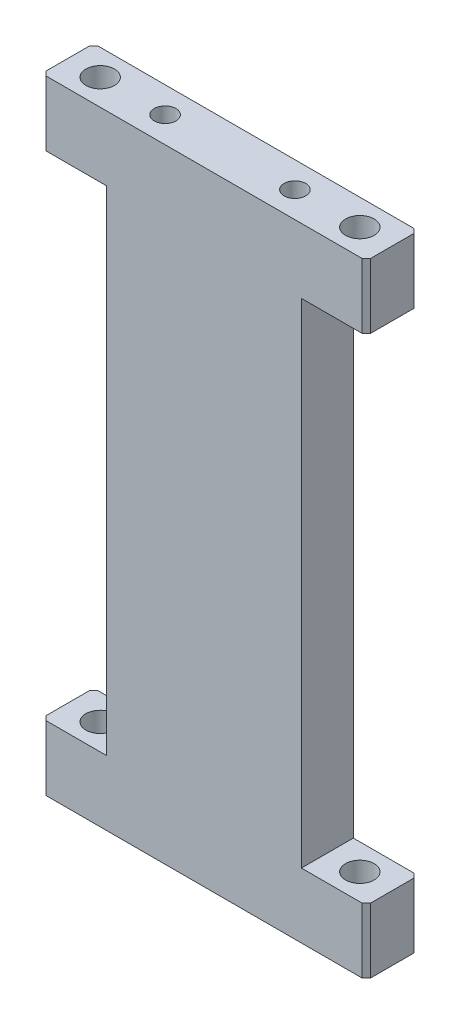
SolidWorks part; units mm, degrees
material "AL6061"
ref_plane "Front Plane" through (0, 0, 0) normal (0, 0, 1) x (1, 0, 0)
ref_plane "Top Plane" through (0, 0, 0) normal (0, 1, 0) x (1, 0, 0)
ref_plane "Right Plane" through (0, 0, 0) normal (1, 0, 0) x (0, 0, -1)
sketch "Sketch1" plane through (0, 0, 0) normal (0, 0, 1) x (1, 0, 0)
  line L1 (-37.5, 72) -> (37.5, 72)
  line L2 (-37.5, 72) -> (-37.5, -72)
  line L3 (-37.5, -72) -> (37.5, -72)
  line L4 (37.5, 72) -> (37.5, -72)
  line L5 (-37.5, 72) -> (37.5, -72) construction
  line L6 (-37.5, -72) -> (37.5, 72) construction
  point P0 (0, 0)
  dimension "D1" = 144
  dimension "D2" = 75
extrude "Boss-Extrude1" add sketch "Sketch1" along normal mid plane 12
sketch "Sketch4" plane through (0, 0, 6) normal (0, 0, 1) x (1, 0, 0)
  line L0 (-37.5, 72) -> (-37.5, -72) construction
  line L1 (-37.5, 57) -> (-22.5, 57)
  line L2 (-37.5, 57) -> (-37.5, -57)
  line L3 (-37.5, -57) -> (-22.5, -57)
  line L4 (-22.5, 57) -> (-22.5, -57)
  line L5 (-37.5, 57) -> (-22.5, -57) construction
  line L6 (-37.5, -57) -> (-22.5, 57) construction
  line L7 (37.5, 72) -> (-37.5, 72) construction
  line L8 (-37.5, -72) -> (37.5, -72) construction
  point P0 (-30, 0)
  dimension "D1" = 15
  dimension "D2" = 15
  dimension "D3" = 15
extrude "Cut-Extrude1" cut sketch "Sketch4" against normal through all
mirror "Mirror1" about plane through (0, 0, 0) normal (1, 0, 0) of "Cut-Extrude1"
hole_wizard "Ø6.6 (6.6) Diameter Hole1" positions "Sketch5" profile "Sketch6" hole size "Ø6.6" standard "ISO" end condition through all
sketch "Sketch5" plane through (0, -72, 0) normal (0, -1, 0) x (-1, 0, 0)
  line L0 (0, 0) -> (0, -27.9261) construction
  line L3 (-37.5, -6) -> (-37.5, 6) construction
  point P0 (-30, 0)
  point P2 (30, 0)
  dimension "D1" = 7.5
sketch "Sketch6" plane through (30, -72, 0) normal (1, 0, 0) x (0, 0, -1)
  line L0 (0, 0) -> (0, 144)
  line L1 (0, 144) -> (3.3, 144)
  line L2 (3.3, 144) -> (3.3, 0)
  line L5 (3.3, 0) -> (0, 0)
  line L11 (0, -6.35) -> (0, 107.95) construction
  dimension "通孔孔直径" = 6.6
  dimension "通孔孔深度" = 144
hole_wizard "Blind Pin Hole1 (size mm)" positions "Sketch7" profile "Sketch8" hole size "Ø5.0" standard "ISO"
sketch "Sketch7" plane through (0, -72, 0) normal (0, -1, 0) x (-1, 0, 0)
  point P0 (-15, 0)
  point P3 (15, 0)
sketch "Sketch8" plane through (15, -72, 0) normal (1, 0, 0) x (0, 0, -1)
  line L0 (0, 0) -> (0, 12.5022)
  line L1 (0, 12.5022) -> (2.5, 11)
  line L2 (2.5, 11) -> (2.5, 0)
  line L5 (2.5, 0) -> (0, 0)
  line L10 (0, 12.5022) -> (-2.5, 11) construction
  line L11 (0, -6.35) -> (0, 107.95) construction
  dimension "孔直径" = 5
  dimension "孔深度" = 11
  dimension "导头角度" = 118
mirror "Mirror2" about plane through (0, 0, 0) normal (0, 1, 0) of "Blind Pin Hole1 (size mm)"
chamfer "Chamfer1" distance 1 angle 45 8 edges at (37.5, -64.5, -6) (37.5, -64.5, 6) (-37.5, -64.5, 6) (-37.5, -64.5, -6) (-37.5, 64.5, -6) (-37.5, 64.5, 6) (37.5, 64.5, 6) (37.5, 64.5, -6)
